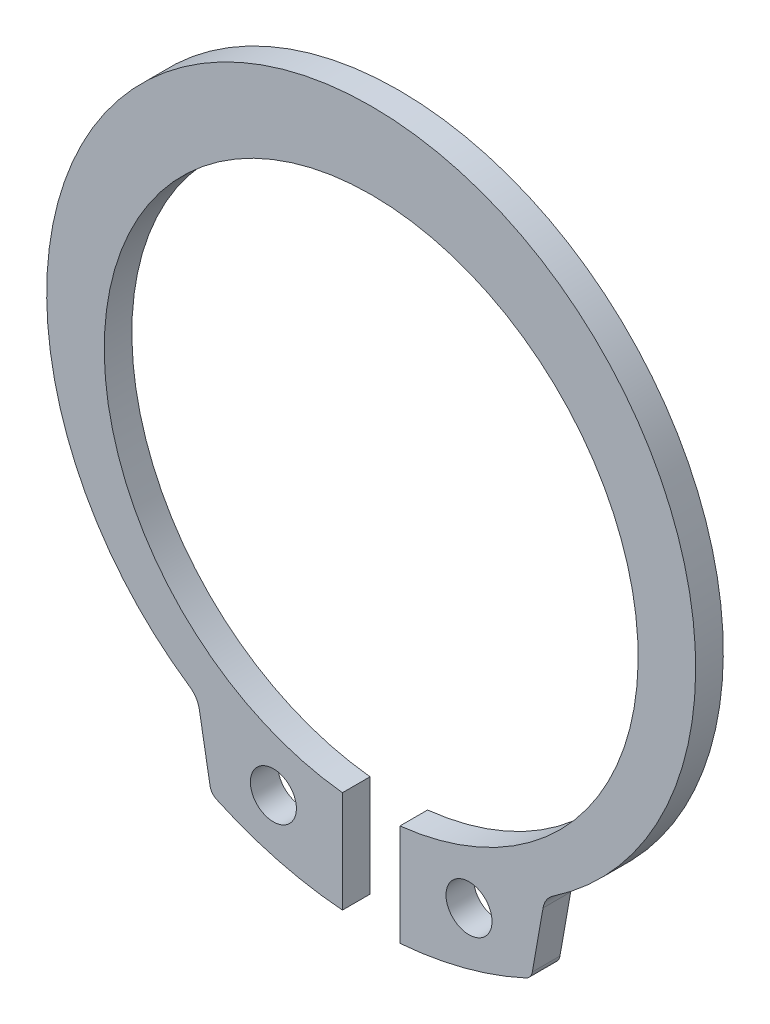
SolidWorks part; units mm, degrees
ref_plane "前视基准面" through (0, 0, 0) normal (0, 0, 1) x (1, 0, 0)
ref_plane "上视基准面" through (0, 0, 0) normal (0, 1, 0) x (1, 0, 0)
ref_plane "右视基准面" through (0, 0, 0) normal (1, 0, 0) x (0, 0, -1)
ref_plane "基准面4" through (0, 0, -1.2) normal (0, 0, -1) x (-1, 0, 0)
sketch "草图1" plane through (0, 0, -1.2) normal (0, 0, -1) x (-1, 0, 0)
  line L0 (-1.25, -16.7811) -> (-1.25, -12.3625)
  line L1 (1.25, -12.3625) -> (1.25, -16.7811)
  line L2 (7.0017, -14.9838) -> (7.4681, -12.3387)
  line L3 (-7.4681, -12.3387) -> (-7.0017, -14.9838)
  circle A0 centre (-4.25, -13.9593) radius 1
  circle A1 centre (4.25, -13.9593) radius 1
  arc A2 (-1.25, -12.3625) -> (1.25, -12.3625) centre (0, -0.83) cw
  arc A3 (1.25, -16.7811) -> (6.7193, -15.3507) centre (0, -0.83) ccw
  arc A4 (6.7193, -15.3507) -> (7.0017, -14.9838) centre (6.5093, -14.897) ccw
  arc A5 (7.4681, -12.3387) -> (7.8931, -11.6837) centre (8.4529, -12.5123) cw
  arc A6 (7.8931, -11.6837) -> (-7.8931, -11.6837) centre (0, 0) ccw
  arc A7 (-7.8931, -11.6837) -> (-7.4681, -12.3387) centre (-8.4529, -12.5123) cw
  arc A8 (-7.0017, -14.9838) -> (-6.7193, -15.3507) centre (-6.5093, -14.897) ccw
  arc A9 (-6.7193, -15.3507) -> (-1.25, -16.7811) centre (0, -0.83) ccw
extrude "凸台-拉伸1" add sketch "草图1" against normal blind 1.2
